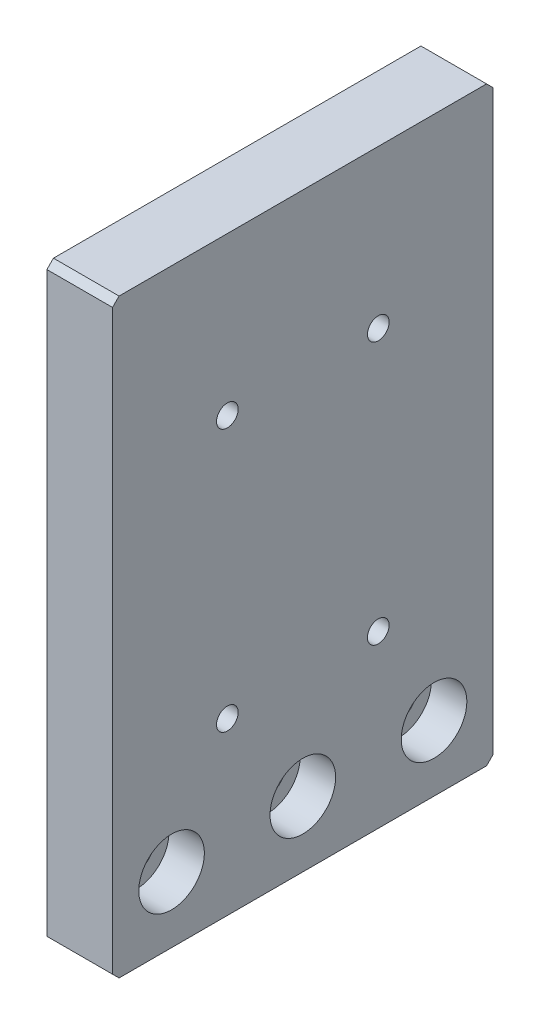
SolidWorks part; units mm, degrees
material "Al6061"
ref_plane "Front" through (0, 0, 0) normal (0, 0, 1) x (1, 0, 0)
ref_plane "Top" through (0, 0, 0) normal (0, 1, 0) x (1, 0, 0)
ref_plane "Right" through (0, 0, 0) normal (1, 0, 0) x (0, 0, -1)
sketch "草图1" plane through (0, 0, 0) normal (1, 0, 0) x (0, 0, -1)
  line L1 (-29, 45) -> (29, 45)
  line L2 (-29, 45) -> (-29, -45)
  line L3 (-29, -45) -> (29, -45)
  line L4 (29, 45) -> (29, -45)
  line L5 (-29, 45) -> (29, -45) construction
  line L6 (-29, -45) -> (29, 45) construction
  point P0 (0, 0)
  dimension "D1" = 58
  dimension "D2" = 90
extrude "凸台-拉伸1" add sketch "草图1" along normal blind 10
hole_wizard "M4 螺纹孔1" positions "草图3" profile "草图2" tap size "M4" standard "Iso" end condition through all
sketch "草图3" plane through (10, 0, 0) normal (1, 0, 0) x (0, 0, -1)
  line L0 (0, 0) -> (0, -45) construction
  line L1 (-29, -45) -> (29, -45) construction
  point P0 (-11.5, 21)
  point P2 (11.5, 21)
  point P4 (-11.5, -19)
  point P6 (11.5, -19)
  dimension "D1" = 23
  dimension "D2" = 40
  dimension "D3" = 26
sketch "草图2" plane through (10, 21, 11.5) normal (0, 1, 0) x (0, 0, -1)
  line L0 (0, 0) -> (0, 10)
  line L1 (0, 10) -> (1.65, 10)
  line L2 (1.65, 10) -> (1.65, 0)
  line L5 (1.65, 0) -> (0, 0)
  line L11 (0, -6.35) -> (0, 107.95) construction
  dimension "通孔螺纹孔钻头直径" = 3.3
  dimension "通孔螺纹孔钻头深度" = 10
cosmetic thread "孔螺蚊线1"
cosmetic thread "孔螺蚊线2"
cosmetic thread "孔螺蚊线3"
cosmetic thread "孔螺蚊线4"
hole_wizard "M5 六角凹头螺钉的柱形沉头孔1" positions "草图5" profile "草图4" counterbore size "M5" standard "Iso" end condition through all
sketch "草图5" plane through (10, 0, 0) normal (1, 0, 0) x (0, 0, -1)
  line L0 (0, 0) -> (0, -35) construction
  line L2 (-29, -45) -> (29, -45) construction
  point P0 (-20, -35)
  point P2 (0, -35)
  point P4 (20, -35)
  dimension "D1" = 40
  dimension "D2" = 10
sketch "草图4" plane through (10, -35, 20) normal (0, 1, 0) x (0, 0, -1)
  line L0 (0, 0) -> (0, 10)
  line L1 (0, 10) -> (2.75, 10)
  line L3 (2.75, 10) -> (2.75, 5.4)
  line L4 (2.75, 5.4) -> (5, 5.4)
  line L5 (5, 5.4) -> (5, 0)
  line L7 (5, 0) -> (0, 0)
  line L11 (0, -6.35) -> (0, 107.95) construction
  dimension "通孔孔直径" = 5.5
  dimension "通孔孔深度" = 10
  dimension "柱形沉头孔直径" = 10
  dimension "柱形沉头孔深度" = 5.4
chamfer "倒角1" distance 1 angle 45 4 edges at (5, -45, -29) (5, -45, 29) (5, 45, -29) (5, 45, 29)
